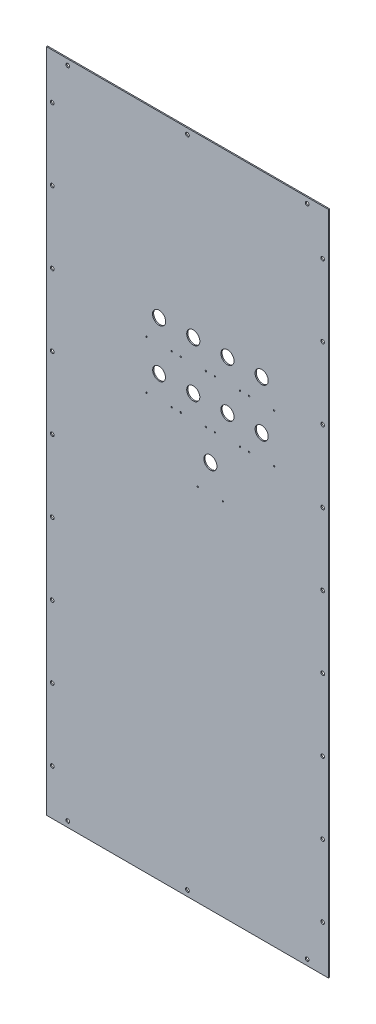
from build123d import *

# Parameters (mm, degrees)
SKETCH_1_W          = 494.5
SKETCH_1_H          = 1168
SKETCH_1_R          = 3.25
EXTRUDE_1_DEPTH     = 2
SKETCH_3_R          = 1.15
SKETCH_3_R_2        = 11.5
SKETCH_3_R_3        = 11.25
CUT_EXTRUDE_2_DEPTH = 10


with BuildPart() as part:
    # 草图1 → 凸台-拉伸1 (new body)
    with BuildSketch(Plane.XY):
        Rectangle(SKETCH_1_W, SKETCH_1_H)
        with Locations((-237.25, 0)):
            Circle(SKETCH_1_R, mode=Mode.SUBTRACT)
        with Locations((-237.25, -126)):
            Circle(SKETCH_1_R, mode=Mode.SUBTRACT)
        with Locations((-237.25, -252)):
            Circle(SKETCH_1_R, mode=Mode.SUBTRACT)
        with Locations((-237.25, -378)):
            Circle(SKETCH_1_R, mode=Mode.SUBTRACT)
        with Locations((-237.25, -504)):
            Circle(SKETCH_1_R, mode=Mode.SUBTRACT)
        with Locations((0, -574)):
            Circle(SKETCH_1_R, mode=Mode.SUBTRACT)
        with Locations(Location((0, 574, 0), (0, 0, 180))):
            Circle(SKETCH_1_R, mode=Mode.SUBTRACT)
        with Locations(Location((-237.25, 504, 0), (0, 0, 180))):
            Circle(SKETCH_1_R, mode=Mode.SUBTRACT)
        with Locations(Location((-237.25, 378, 0), (0, 0, 180))):
            Circle(SKETCH_1_R, mode=Mode.SUBTRACT)
        with Locations(Location((-237.25, 252, 0), (0, 0, 180))):
            Circle(SKETCH_1_R, mode=Mode.SUBTRACT)
        with Locations(Location((-237.25, 126, 0), (0, 0, 180))):
            Circle(SKETCH_1_R, mode=Mode.SUBTRACT)
        with Locations((237.25, 126)):
            Circle(SKETCH_1_R, mode=Mode.SUBTRACT)
        with Locations((237.25, 252)):
            Circle(SKETCH_1_R, mode=Mode.SUBTRACT)
        with Locations((237.25, 378)):
            Circle(SKETCH_1_R, mode=Mode.SUBTRACT)
        with Locations((237.25, 504)):
            Circle(SKETCH_1_R, mode=Mode.SUBTRACT)
        with Locations(Location((237.25, -504, 0), (0, 0, 180))):
            Circle(SKETCH_1_R, mode=Mode.SUBTRACT)
        with Locations(Location((237.25, -378, 0), (0, 0, 180))):
            Circle(SKETCH_1_R, mode=Mode.SUBTRACT)
        with Locations(Location((237.25, -252, 0), (0, 0, 180))):
            Circle(SKETCH_1_R, mode=Mode.SUBTRACT)
        with Locations(Location((237.25, -126, 0), (0, 0, 180))):
            Circle(SKETCH_1_R, mode=Mode.SUBTRACT)
        with Locations(Location((237.25, 0, 0), (0, 0, 180))):
            Circle(SKETCH_1_R, mode=Mode.SUBTRACT)
        with Locations((-210, 574)):
            Circle(SKETCH_1_R, mode=Mode.SUBTRACT)
        with Locations((210, 574)):
            Circle(SKETCH_1_R, mode=Mode.SUBTRACT)
        with Locations(Location((210, -574, 0), (0, 0, 180))):
            Circle(SKETCH_1_R, mode=Mode.SUBTRACT)
        with Locations(Location((-210, -574, 0), (0, 0, 180))):
            Circle(SKETCH_1_R, mode=Mode.SUBTRACT)
    extrude(amount=EXTRUDE_1_DEPTH)

    # 草图3 → 切除-拉伸2 (cut)
    with BuildSketch(Plane(origin=(0, 0, 0), x_dir=(-1, 0, 0), z_dir=(0, 0, -1))):
        with Locations((-48.25, 145.832522251)):
            Circle(SKETCH_3_R)
        with Locations((-10.25, 185.832522251)):
            Circle(SKETCH_3_R_2)
        with Locations((-32.25, 145.832522251)):
            Circle(SKETCH_3_R)
        with Locations((11.75, 145.832522251)):
            Circle(SKETCH_3_R)
        with Locations((27.75, 145.832522251)):
            Circle(SKETCH_3_R)
        with Locations((71.75, 145.832522251)):
            Circle(SKETCH_3_R)
        with Locations((49.75, 270.832522251)):
            Circle(SKETCH_3_R_2)
        with Locations((27.75, 230.832522251)):
            Circle(SKETCH_3_R)
        with Locations((71.75, 230.832522251)):
            Circle(SKETCH_3_R)
        with Locations((-130.25, 185.832522251)):
            Circle(SKETCH_3_R_2)
        with Locations((-152.25, 145.832522251)):
            Circle(SKETCH_3_R)
        with Locations((-108.25, 145.832522251)):
            Circle(SKETCH_3_R)
        with Locations((-70.25, 185.832522251)):
            Circle(SKETCH_3_R_2)
        with Locations((-92.25, 145.832522251)):
            Circle(SKETCH_3_R)
        with Locations((-152.25, 230.832522251)):
            Circle(SKETCH_3_R)
        with Locations((-108.25, 230.832522251)):
            Circle(SKETCH_3_R)
        with Locations((-70.25, 270.832522251)):
            Circle(SKETCH_3_R_2)
        with Locations((-92.25, 230.832522251)):
            Circle(SKETCH_3_R)
        with Locations((-48.25, 230.832522251)):
            Circle(SKETCH_3_R)
        with Locations((-10.25, 270.832522251)):
            Circle(SKETCH_3_R_2)
        with Locations((-32.25, 230.832522251)):
            Circle(SKETCH_3_R)
        with Locations((11.75, 230.832522251)):
            Circle(SKETCH_3_R)
        with Locations((-40.25, 95.832522251)):
            Circle(SKETCH_3_R_2)
        with Locations((-62.25, 47.832522251)):
            Circle(SKETCH_3_R)
        with Locations((-18.25, 47.832522251)):
            Circle(SKETCH_3_R)
        with Locations((-130.25, 270.832522251)):
            Circle(SKETCH_3_R_2)
        with Locations((49.75, 185.832522251)):
            Circle(SKETCH_3_R_3)
    extrude(amount=-CUT_EXTRUDE_2_DEPTH, mode=Mode.SUBTRACT)


solid = part.part
